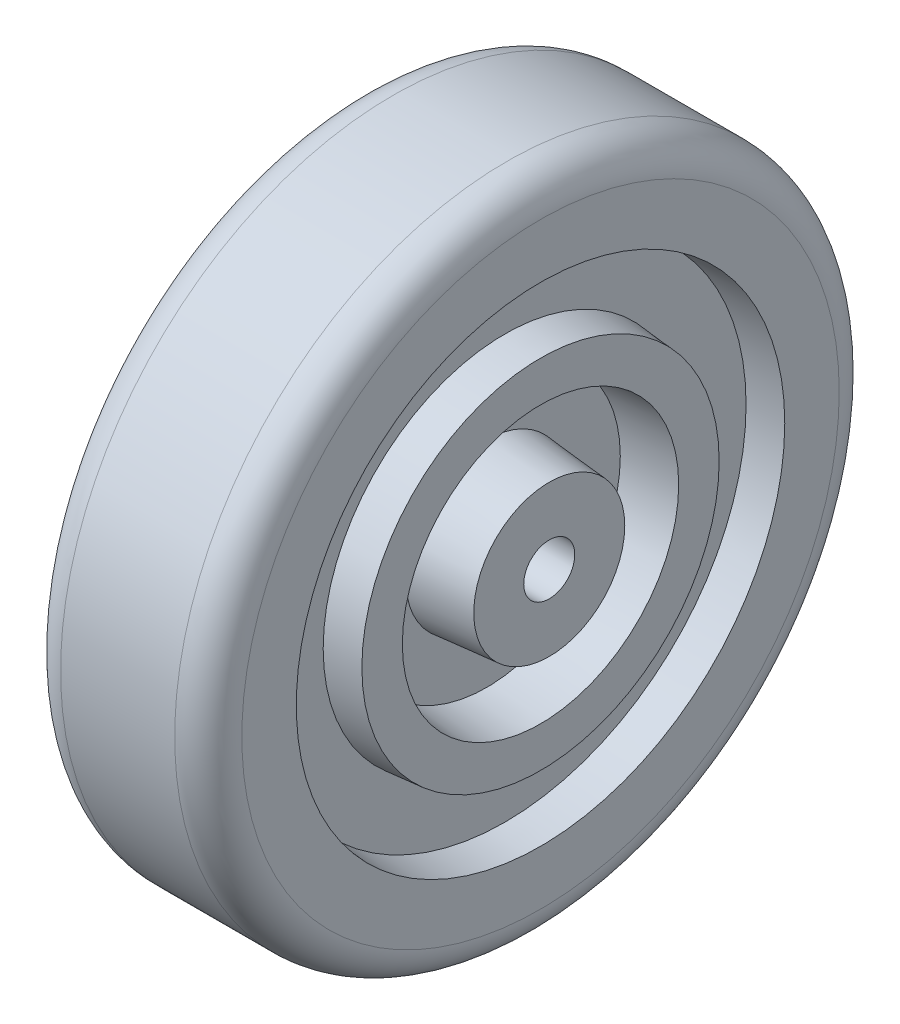
from build123d import *

# Parameters (mm, degrees)
BOSS_EXTRUDE1_DEPTH      = 17.145
BOSS_EXTRUDE1_DEPTH_BACK = 17.145
SKETCH1_R                = 62.865
SKETCH2_R                = 46.355
SKETCH2_R_2              = 33.655
CUT_EXTRUDE1_DEPTH       = 6.731
SKETCH3_R                = 26.289
CUT_EXTRUDE2_DEPTH       = 10.16
BOSS_EXTRUDE2_DEPTH      = 18.796
BOSS_EXTRUDE2_DEPTH_BACK = 18.796
SKETCH4_R                = 14.2875
FILLET1_R                = 6.35
DRAFT1_ANGLE             = 5
DRAFT2_ANGLE             = 5
SKETCH5_R                = 4.826
CUT_EXTRUDE3_DEPTH       = 175.112368419
SKETCH6_W                = 11.857056217
SKETCH6_H                = 6.35
EXTRUDE_THIN1_DEPTH      = 6.35


with BuildPart() as part:
    # Sketch1 → Boss-Extrude1 (new, two sides: drawn at the far end of the back side and taken through both)
    with BuildSketch(Plane(origin=(0, 0, 0), x_dir=(0, 0, -1), z_dir=(1, 0, 0)).offset(-BOSS_EXTRUDE1_DEPTH_BACK)):
        with Locations((34.925, -76.2)):
            Circle(SKETCH1_R)
    extrude(amount=BOSS_EXTRUDE1_DEPTH + BOSS_EXTRUDE1_DEPTH_BACK)

    # Sketch2 → Cut-Extrude1 (cut)
    with BuildSketch(Plane.ZY.offset(17.145)):
        with Locations((-34.925, -76.2)):
            Circle(SKETCH2_R)
        with Locations((-34.925, -76.2)):
            Circle(SKETCH2_R_2, mode=Mode.SUBTRACT)
    cut_extrude1 = extrude(amount=-CUT_EXTRUDE1_DEPTH, mode=Mode.SUBTRACT)

    # Sketch3 → Cut-Extrude2 (cut)
    with BuildSketch(Plane.ZY.offset(17.145)):
        with Locations((-34.925, -76.2)):
            Circle(SKETCH3_R)
    cut_extrude2 = extrude(amount=-CUT_EXTRUDE2_DEPTH, mode=Mode.SUBTRACT)

    # Mirror1: Cut-Extrude1, Cut-Extrude2 across plane
    add(cut_extrude1.mirror(Plane(origin=(0, 0, 0), x_dir=(0, 0, 1), z_dir=(1, 0, 0))), mode=Mode.SUBTRACT)
    add(cut_extrude2.mirror(Plane(origin=(0, 0, 0), x_dir=(0, 0, 1), z_dir=(1, 0, 0))), mode=Mode.SUBTRACT)

    # Sketch4 → Boss-Extrude2 (add, two sides: drawn at the far end of the back side and taken through both)
    with BuildSketch(Plane(origin=(0, 0, 0), x_dir=(0, 0, -1), z_dir=(1, 0, 0)).offset(-BOSS_EXTRUDE2_DEPTH_BACK)):
        with Locations((34.925, -76.2)):
            Circle(SKETCH4_R)
    extrude(amount=BOSS_EXTRUDE2_DEPTH + BOSS_EXTRUDE2_DEPTH_BACK)

    # Fillet1
    fillet1_edges = [part.edges().sort_by_distance(p)[0] for p in [
        (-17.145, -76.2, 27.94),
        (17.145, -76.2, 27.94),
    ]]
    fillet(fillet1_edges, radius=FILLET1_R)

    # Draft1
    draft1_faces = [part.faces().sort_by_distance(p)[0] for p in [
        (-13.7795, -76.2, -81.28),
        (-13.7795, -76.2, -68.58),
        (-12.065, -76.2, -61.214),
        (-12.8905, -76.2, -20.6375),
    ]]
    draft(draft1_faces, Plane(origin=(-18.796, -76.2, -34.925), x_dir=(0, 0, -1), z_dir=(-1, 0, 0)), DRAFT1_ANGLE)

    # Draft2
    draft2_faces = [part.faces().sort_by_distance(p)[0] for p in [
        (13.7795, -76.2, -81.28),
        (13.7795, -76.2, -68.58),
        (12.065, -76.2, -61.214),
        (12.8905, -76.2, -20.6375),
    ]]
    draft(draft2_faces, Plane(origin=(18.796, -76.2, -34.925), x_dir=(0, 0, 1), z_dir=(1, 0, 0)), DRAFT2_ANGLE)

    # Sketch5 → Cut-Extrude3 (cut, through all)
    with BuildSketch(Plane.ZY.offset(18.796)):
        with Locations((-34.925, -76.2)):
            Circle(SKETCH5_R)
    extrude(amount=-CUT_EXTRUDE3_DEPTH, mode=Mode.SUBTRACT)

    # Sketch6 → Extrude-Thin1 (add)
    with BuildSketch(Plane.ZY.offset(6.985)):
        with Locations((-55.141028109, -76.2)):
            Rectangle(SKETCH6_W, SKETCH6_H)
        with Locations((-14.708971892, -76.2)):
            Rectangle(SKETCH6_W, SKETCH6_H)
    extrude(amount=EXTRUDE_THIN1_DEPTH)


solid = part.part
